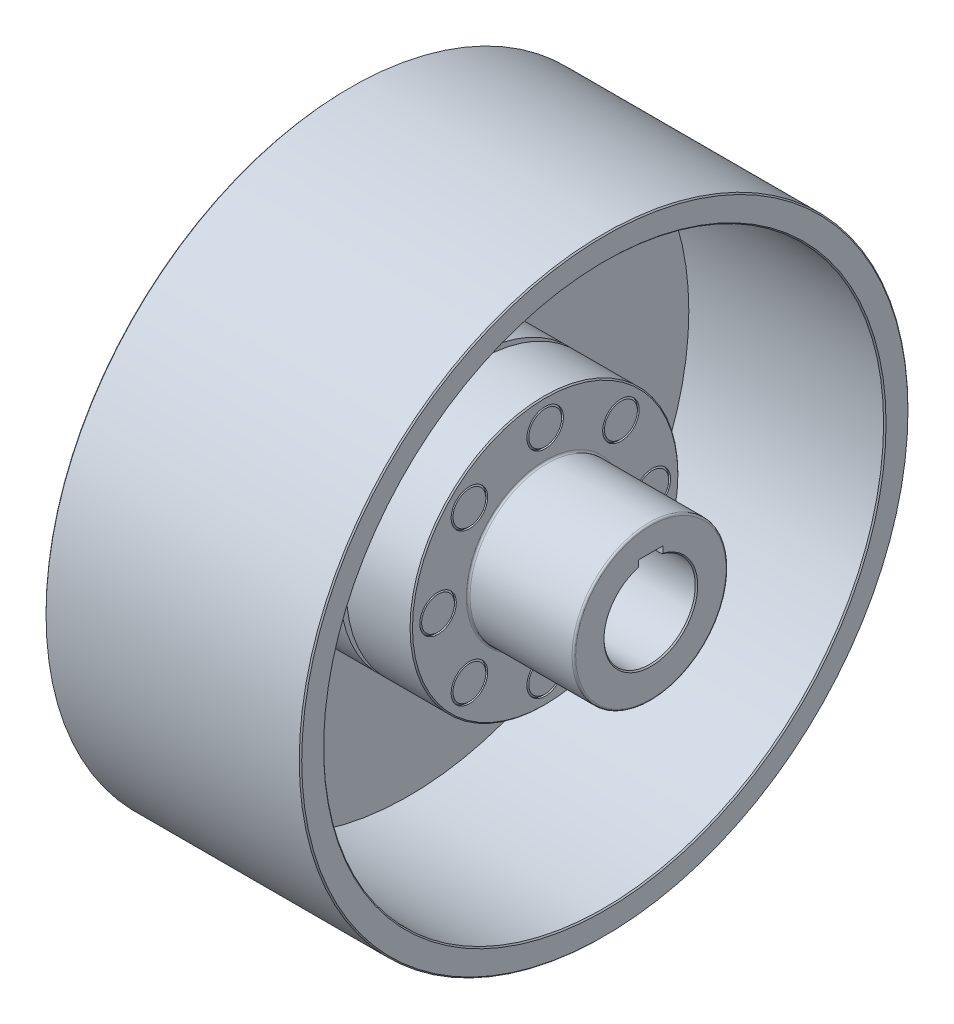
SolidWorks part; units mm, degrees
material "Q235-A (F)"
ref_plane "Front Plane" through (0, 0, 0) normal (0, 0, 1) x (1, 0, 0)
ref_plane "Top Plane" through (0, 0, 0) normal (0, 1, 0) x (1, 0, 0)
ref_plane "Right Plane" through (0, 0, 0) normal (1, 0, 0) x (0, 0, -1)
sketch "Sketch1" plane through (0, 0, 0) normal (0, 0, 1) x (1, 0, 0)
  line L0 (-114.849, 0) -> (199.5633, 0) construction
  line L1 (-2.8, 56.925) -> (-30.8, 56.925)
  line L2 (-30.8, 56.925) -> (-30.8, 37.5)
  line L3 (-30.8, 37.5) -> (-142.8, 37.5)
  line L4 (-142.8, 37.5) -> (-142.8, 63.25)
  line L5 (-142.8, 63.25) -> (-61.6, 63.25)
  line L6 (-56, 68.85) -> (-56, 110)
  line L7 (-56, 110) -> (-2.8, 110)
  line L8 (-2.8, 110) -> (-2.8, 104.5)
  line L9 (2.8, 110) -> (56, 110)
  line L10 (56, 110) -> (56, 63.25)
  line L11 (56, 63.25) -> (142.8, 63.25)
  line L12 (142.8, 63.25) -> (142.8, 37.5)
  line L13 (142.8, 37.5) -> (2.8, 37.5)
  line L14 (2.8, 104.5) -> (2.8, 110)
  line L15 (0, 0) -> (0, 250) construction
  line L16 (-56, 63.25) -> (56, 63.25) construction
  line L17 (-2.8, 56.925) -> (-2.8, 37.5) construction
  line L18 (-2.8, 37.5) -> (-142.8, 37.5) construction
  line L19 (-56, 88) -> (56, 88) construction
  line L20 (-56, 103) -> (-40.6125, 103) construction
  line L21 (-61.6, 63.25) -> (-61.6, 68.85)
  line L22 (-61.6, 68.85) -> (-56, 68.85)
  line L23 (2.8, 110) -> (-2.8, 110) construction
  line L24 (105, 250) -> (-105, 250) construction
  line L25 (-105, 250) -> (-105, 230) construction
  line L26 (-105, 230) -> (-61.6, 230) construction
  line L27 (-61.6, 230) -> (-61.6, 68.85) construction
  line L28 (-56, 230) -> (105, 230) construction
  line L29 (105, 230) -> (105, 250) construction
  line L30 (-56, 230) -> (-56, 110) construction
  line L31 (2.8, 37.5) -> (2.8, 0)
  line L32 (2.8, 0) -> (-2.8, 0)
  line L33 (-2.8, 0) -> (-2.8, 56.925)
  line L34 (-2.8, 104.5) -> (2.8, 104.5)
  dimension "L" = 112
  dimension "D" = 220
  dimension "D7" = 176
  dimension "d2" = 75
  dimension "D3" = 30
  dimension "d1" = 75
  dimension "D4" = 126.5
  dimension "D5" = 113.85
  dimension "D6" = 5.6
  dimension "D8" = 460
  dimension "D0" = 500
  dimension "B" = 210
  dimension "D9" = 209
  dimension "D10" = 140
  dimension "D11" = 28
  dimension "D12" = 140
revolve "Revolve1" add sketch "Sketch1" angle 360 about L0
sketch "Sketch2" plane through (0, 0, 0) normal (0, 0, 1) x (1, 0, 0)
  line L0 (105, 250) -> (-105, 250)
  line L1 (-105, 250) -> (-105, 230)
  line L2 (-105, 230) -> (-61.6, 230)
  line L3 (-61.6, 230) -> (-61.6, 68.85)
  line L4 (-61.6, 68.85) -> (-56, 68.85)
  line L5 (-56, 68.85) -> (-56, 230)
  line L6 (-56, 230) -> (105, 230)
  line L7 (105, 230) -> (105, 250)
  line L8 (0, 0) -> (-89.3526, 0) construction
  line L9 (-114.849, 0) -> (199.5633, 0) construction
revolve "Revolve2" add sketch "Sketch2" angle 360 about L8
sketch "Sketch3" plane through (0, 0, 0) normal (0, 0, 1) x (1, 0, 0)
  line L0 (-56, 103) -> (-61.6, 103)
  line L2 (-61.6, 230) -> (-61.6, 68.85) construction
  line L3 (-61.6, 103) -> (-61.6, 88)
  line L5 (-61.6, 88) -> (-56, 88)
  line L7 (-56, 88) -> (-56, 101.5)
  line L8 (-56, 68.85) -> (-56, 110) construction
  line L9 (-56, 101.5) -> (-54.5, 103)
  line L10 (-56, 103) -> (-40.6125, 103) construction
  line L11 (-56, 103) -> (-54.5, 103)
  line L12 (56, 103) -> (54.5, 103)
  line L13 (56, 110) -> (56, 63.25) construction
  line L14 (54.5, 103) -> (56, 101.5)
  line L15 (56, 101.5) -> (56, 103)
  dimension "D1" = 45
  dimension "D2" = 1.5
revolve "Cut-Revolve1" cut sketch "Sketch3" angle 360 about L5
chamfer "Chamfer1" distance 1 angle 45 2 edges at (56, 0, 110) (142.8, 0, 37.5)
chamfer "Chamfer2" distance 1 angle 45 4 edges at (-105, 0, -250) (-105, 0, -230) (105, 0, -230) (105, 0, -250)
chamfer "Chamfer3" distance 1 angle 45 1 edges at (-142.8, 0, 37.5)
fillet "Fillet1" radius 1.5 2 edges at (-61.6, 0, 63.25) (-142.8, 0, 63.25)
fillet "Fillet2" radius 1.5 2 edges at (142.8, 0, 63.25) (56, 0, 63.25)
sketch "Sketch5" plane through (-61.6, 0, 0) normal (-1, 0, 0) x (0, 0, 1)
  line L0 (0, 88) -> (0, 0) construction
  line L1 (33.6761, 76.9713) -> (37.4261, 79.1363)
  line L2 (37.4261, 79.1363) -> (37.4261, 83.4665)
  line L3 (37.4261, 83.4665) -> (33.6761, 85.6315)
  line L4 (33.6761, 85.6315) -> (29.9261, 83.4665)
  line L5 (29.9261, 83.4665) -> (29.9261, 79.1363)
  line L6 (29.9261, 79.1363) -> (33.6761, 76.9713)
  line L7 (0, 0) -> (33.6761, 81.3014) construction
  circle A0 centre (0, 0) radius 88 construction
  circle A1 centre (33.6761, 81.3014) radius 3.75 construction
  dimension "D2" = 7.5
  dimension "D1" = 22.5
extrude "Extrude1" add sketch "Sketch5" along normal blind 3.375
pattern_circular "CirPattern11" count 8 over 360 about axis through (0, 0, 0) along (1, 0, 0) of "Cut-Revolve1", "Extrude1"
sketch "Sketch6" plane through (142.8, 0, 0) normal (1, 0, 0) x (0, 0, -1)
  line L1 (-10, 42.4) -> (10, 42.4)
  line L2 (-10, 42.4) -> (-10, 32.6)
  line L3 (-10, 32.6) -> (10, 32.6)
  line L4 (10, 42.4) -> (10, 32.6)
  line L5 (-10, 42.4) -> (10, 32.6) construction
  line L6 (-10, 32.6) -> (10, 42.4) construction
  circle A0 centre (0, 0) radius 37.5 construction
  point P0 (0, 37.5)
  dimension "D1" = 20
  dimension "D2" = 4.9
extrude "Cut-Extrude1" cut sketch "Sketch6" against normal through all
